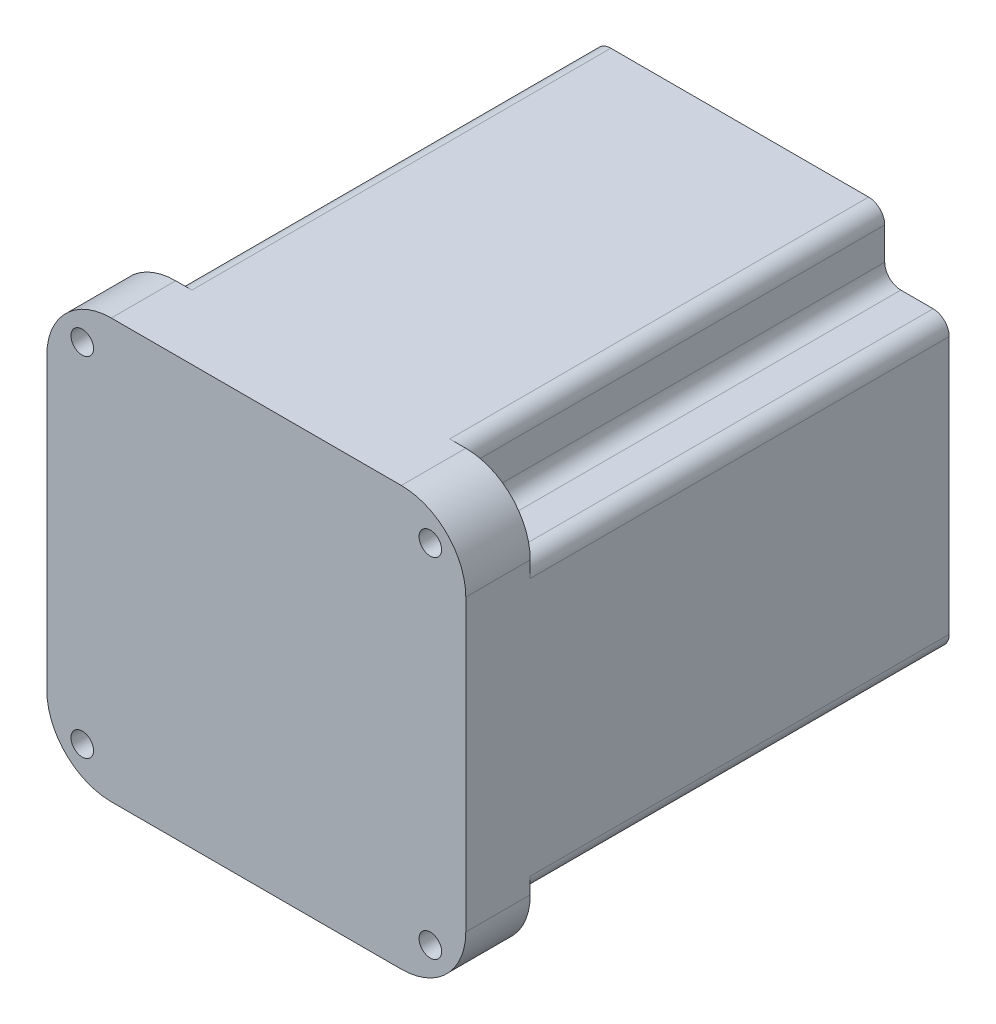
from build123d import *

# Parameters (mm, degrees)
SKETCH1_W           = 130
SKETCH1_H           = 130
BOSS_EXTRUDE1_DEPTH = 150
FILLET1_R           = 20
SKETCH2_W           = 69.063294878
SKETCH2_H           = 85.712482036
CUT_EXTRUDE1_DEPTH  = 130
CIRPATTERN1_COUNT   = 4
FILLET2_R           = 5
FILLET3_R           = 5
SKETCH4_R           = 3.5
CUT_EXTRUDE2_DEPTH  = 40
CIRPATTERN2_COUNT   = 4


with BuildPart() as part:
    # Sketch1 → Boss-Extrude1 (new body)
    with BuildSketch(Plane.XY):
        Rectangle(SKETCH1_W, SKETCH1_H)
    extrude(amount=BOSS_EXTRUDE1_DEPTH)

    # Fillet1
    fillet1_edges = [part.edges().sort_by_distance(p)[0] for p in [
        (65, -65, 75),
        (-65, -65, 75),
        (-65, 65, 75),
        (65, 65, 75),
    ]]
    fillet(fillet1_edges, radius=FILLET1_R)

    # Sketch2 → Cut-Extrude1 (cut)
    with BuildSketch(Plane(origin=(0, 0, 0), x_dir=(-1, 0, 0), z_dir=(0, 0, -1))):
        with Locations((-79.531647439, 87.856241018)):
            Rectangle(SKETCH2_W, SKETCH2_H)
    cut_extrude1 = extrude(amount=-CUT_EXTRUDE1_DEPTH, mode=Mode.SUBTRACT)

    # CirPattern1: Cut-Extrude1 ×4 about axis
    cirpattern1_axis = Axis((0, 0, 0), (0, 0, 1))
    for i in range(1, CIRPATTERN1_COUNT):
        add(cut_extrude1.rotate(cirpattern1_axis, i * 360 / CIRPATTERN1_COUNT), mode=Mode.SUBTRACT)

    # Fillet2
    fillet2_edges = [part.edges().sort_by_distance(p)[0] for p in [
        (45, 45, 65),
        (-45, 45, 65),
        (-45, -45, 65),
        (45, -45, 65),
    ]]
    fillet(fillet2_edges, radius=FILLET2_R)

    # Fillet3
    fillet3_edges = [part.edges().sort_by_distance(p)[0] for p in [
        (45, -65, 65),
        (-65, -45, 65),
        (65, 45, 65),
        (-45, 65, 65),
        (45, 65, 65),
        (-65, 45, 65),
        (65, -45, 65),
        (-45, -65, 65),
    ]]
    fillet(fillet3_edges, radius=FILLET3_R)

    # Sketch4 → Cut-Extrude2 (cut)
    with BuildSketch(Plane(origin=(0, 0, 130), x_dir=(-1, 0, 0), z_dir=(0, 0, -1))):
        with Locations((54, 54)):
            Circle(SKETCH4_R)
    cut_extrude2 = extrude(amount=-CUT_EXTRUDE2_DEPTH, mode=Mode.SUBTRACT)

    # CirPattern2: Cut-Extrude2 ×4 about axis
    cirpattern2_axis = Axis((0, 0, 0), (0, 0, 1))
    for i in range(1, CIRPATTERN2_COUNT):
        add(cut_extrude2.rotate(cirpattern2_axis, i * 360 / CIRPATTERN2_COUNT), mode=Mode.SUBTRACT)


solid = part.part
